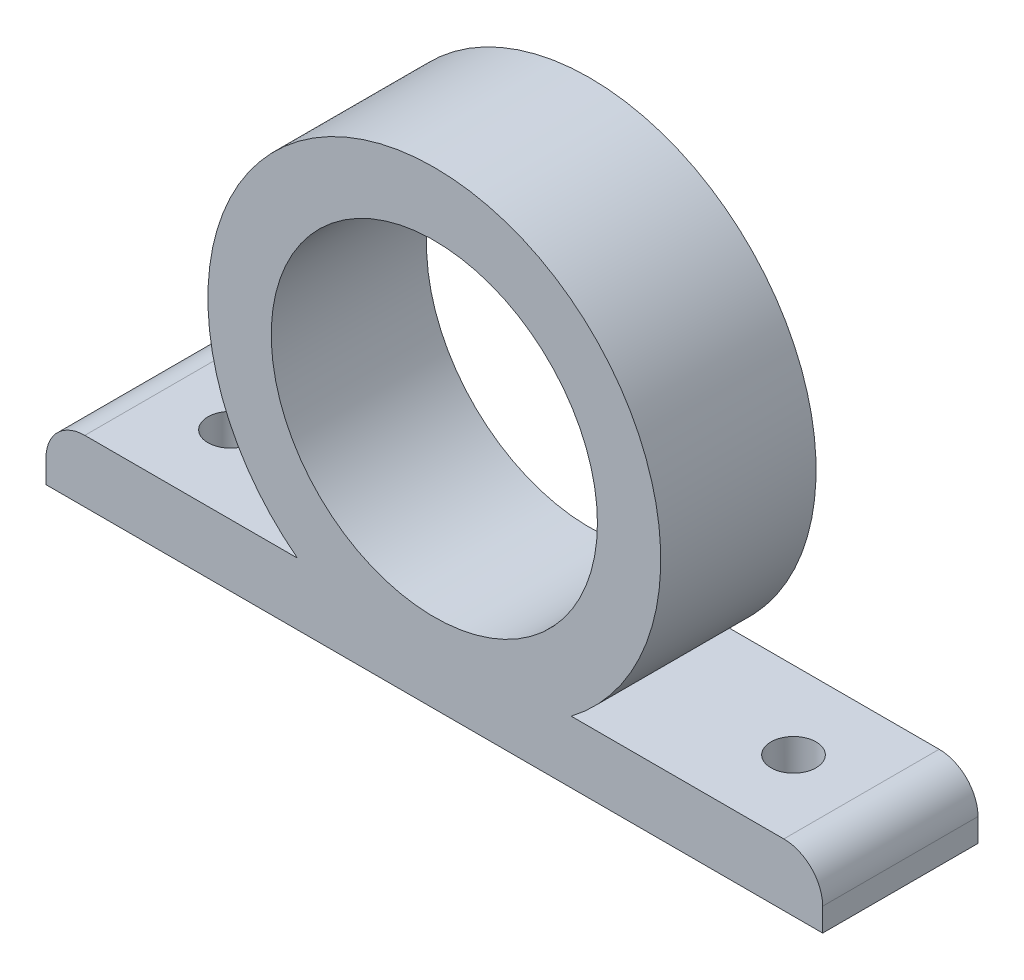
SolidWorks part; units mm, degrees
ref_plane "Front Plane" through (0, 0, 0) normal (0, 0, 1) x (1, 0, 0)
ref_plane "Top Plane" through (0, 0, 0) normal (0, 1, 0) x (1, 0, 0)
ref_plane "Right Plane" through (0, 0, 0) normal (1, 0, 0) x (0, 0, -1)
sketch "Sketch1" plane through (0, 0, 0) normal (0, 1, 0) x (1, 0, 0)
  line L1 (-50, 10) -> (50, 10)
  line L2 (-50, 10) -> (-50, -10)
  line L3 (-50, -10) -> (50, -10)
  line L4 (50, 10) -> (50, -10)
  line L5 (-50, 10) -> (50, -10) construction
  line L6 (-50, -10) -> (50, 10) construction
  point P0 (0, 0)
  dimension "D1" = 100
  dimension "D2" = 20
extrude "Boss-Extrude1" add sketch "Sketch1" along normal blind 8
fillet "Fillet1" radius 5 2 edges at (-50, 8, 0) (50, 8, 0)
sketch "Sketch2" plane through (0, 0, 10) normal (0, 0, 1) x (1, 0, 0)
  line L2 (0, 0) -> (0, 36.6789) construction
  line L3 (-50, 0) -> (50, 0) construction
  circle A0 centre (0, 31.2264) radius 29.1544
  circle A1 centre (0, 31.2264) radius 23.5
  dimension "D2" = 47
extrude "Boss-Extrude3" add sketch "Sketch2" against normal up to surface (20 mm away) up to face at (0, 4.0118, -10)
sketch "Sketch3" plane through (0, 8, 0) normal (0, 1, 0) x (1, 0, 0)
  line L0 (0, 13.9539) -> (0, -17.6711) construction
  circle A0 centre (-36.2466, 0) radius 2.9
  circle A1 centre (36.2466, 0) radius 2.9
  dimension "D1" = 5.8
extrude "Cut-Extrude1" cut sketch "Sketch3" against normal blind 26
sketch "Sketch4" plane through (0, 0, 10) normal (0, 0, 1) x (1, 0, 0)
  circle A0 centre (0, 31.2264) radius 21
  dimension "D1" = 42
extrude "Cut-Extrude2" cut sketch "Sketch4" against normal blind 74
